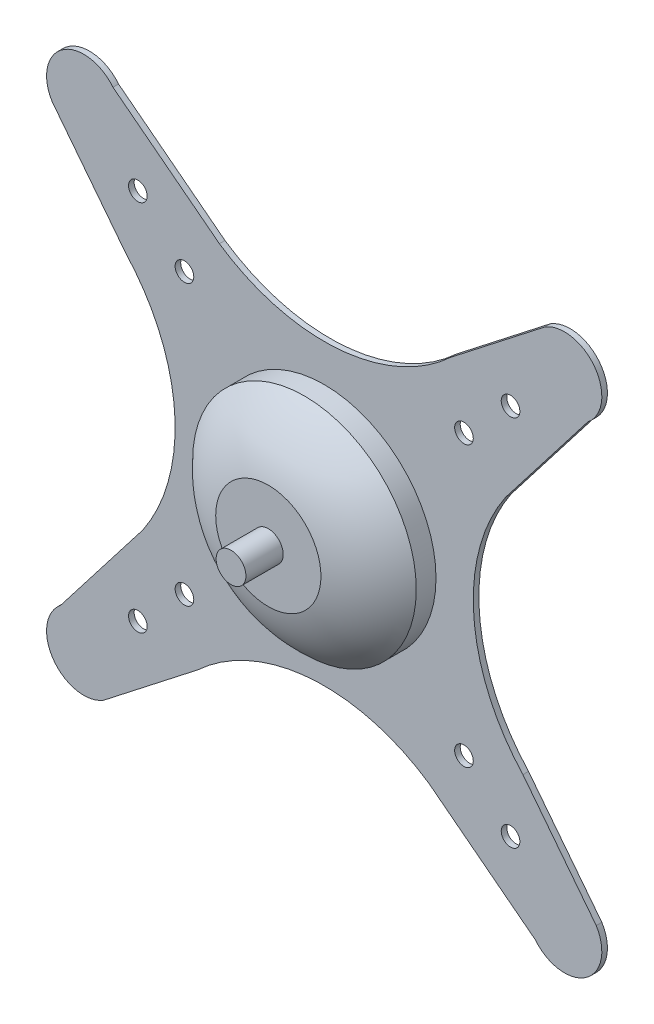
from build123d import *

# Parameters (mm, degrees)
EXTRUDE_1_DEPTH     = 1.5
SKETCH_4_R          = 2.5
CUT_EXTRUDE_1_DEPTH = 1.5
SKETCH_5_R          = 30
EXTRUDE_2_DEPTH     = 15
SKETCH_10_R         = 4
EXTRUDE_3_DEPTH     = 10


with BuildPart() as part:
    # 草图1 → 凸台-拉伸1 (new body)
    with BuildSketch(Plane.XY):
        with BuildLine():
            ThreePointArc((-28.118568833, 48.655761142), (-14.710337472, 42.212909992), (0, 40))
            ThreePointArc((0, 40), (18.246546062, 43.448270099), (33.976331356, 53.317457727))
            Line((33.976331356, 53.317457727), (59.220103302, 72.989737675))
            ThreePointArc((59.220103302, 72.989737675), (72.664625967, 70.256318884), (70.727374666, 56.674204713))
            Line((70.727374666, 56.674204713), (48.655761142, 28.118568833))
            ThreePointArc((48.655761142, 28.118568833), (42.212909992, 14.710337472), (40, 0))
            ThreePointArc((40, 0), (43.448270099, -18.246546062), (53.317457727, -33.976331356))
            Line((53.317457727, -33.976331356), (72.989737675, -59.220103302))
            ThreePointArc((72.989737675, -59.220103302), (70.256318884, -72.664625967), (56.674204713, -70.727374666))
            Line((56.674204713, -70.727374666), (28.118568833, -48.655761142))
            ThreePointArc((28.118568833, -48.655761142), (14.710337472, -42.212909992), (0, -40))
            ThreePointArc((0, -40), (-18.246546062, -43.448270099), (-33.976331356, -53.317457727))
            Line((-33.976331356, -53.317457727), (-59.220103302, -72.989737675))
            ThreePointArc((-59.220103302, -72.989737675), (-72.664625967, -70.256318884), (-70.727374666, -56.674204713))
            Line((-70.727374666, -56.674204713), (-48.655761142, -28.118568833))
            ThreePointArc((-48.655761142, -28.118568833), (-42.212909992, -14.710337472), (-40, 0))
            ThreePointArc((-40, 0), (-43.448270099, 18.246546062), (-53.317457727, 33.976331356))
            Line((-53.317457727, 33.976331356), (-72.989737675, 59.220103302))
            ThreePointArc((-72.989737675, 59.220103302), (-70.256318884, 72.664625967), (-56.674204713, 70.727374666))
            Line((-56.674204713, 70.727374666), (-28.118568833, 48.655761142))
        make_face()
    extrude(amount=EXTRUDE_1_DEPTH)

    # 草图4 → 切除-拉伸1 (cut)
    with BuildSketch(Plane.XY.offset(1.5)):
        with Locations((-50, 50)):
            Circle(SKETCH_4_R)
        with Locations((-37.5, 37.5)):
            Circle(SKETCH_4_R)
        with Locations((50, 50)):
            Circle(SKETCH_4_R)
        with Locations((37.5, 37.5)):
            Circle(SKETCH_4_R)
        with Locations((50, -50)):
            Circle(SKETCH_4_R)
        with Locations((37.5, -37.5)):
            Circle(SKETCH_4_R)
        with Locations((-50, -50)):
            Circle(SKETCH_4_R)
        with Locations((-37.5, -37.5)):
            Circle(SKETCH_4_R)
    extrude(amount=-CUT_EXTRUDE_1_DEPTH, mode=Mode.SUBTRACT)

    # 草图5 → 凸台-拉伸2 (add)
    with BuildSketch(Plane.XY.offset(1.5)):
        Circle(SKETCH_5_R)
    extrude(amount=EXTRUDE_2_DEPTH)

    # 草图6 → 切除-旋转1 (revolve, cut)
    with BuildSketch(Plane(origin=(0, 0, 0), x_dir=(1, 0, 0), z_dir=(0, 1, 0)), mode=Mode.PRIVATE) as cut_revolve_1_sk:
        with BuildLine():
            Line((30, -16.5), (30, -6.799483709))
            add(Edge.make_bspline(
                [(30, -6.799483709), (23.649728085, -14.104545992), (14.118358568, -16.5)],
                knots=[0, 0, 0, 1, 1, 1], degree=2))
            Line((14.118358568, -16.5), (30, -16.5))
        make_face()
    revolve(cut_revolve_1_sk.sketch.rotate(Axis((0, 0, 0), (0, 0, 1)), 180), axis=Axis((0, 0, 0), (0, 0, 1)), mode=Mode.SUBTRACT)

    # 草图10 → 凸台-拉伸3 (add)
    with BuildSketch(Plane.XY.offset(16.5)):
        Circle(SKETCH_10_R)
    extrude(amount=EXTRUDE_3_DEPTH)


solid = part.part
